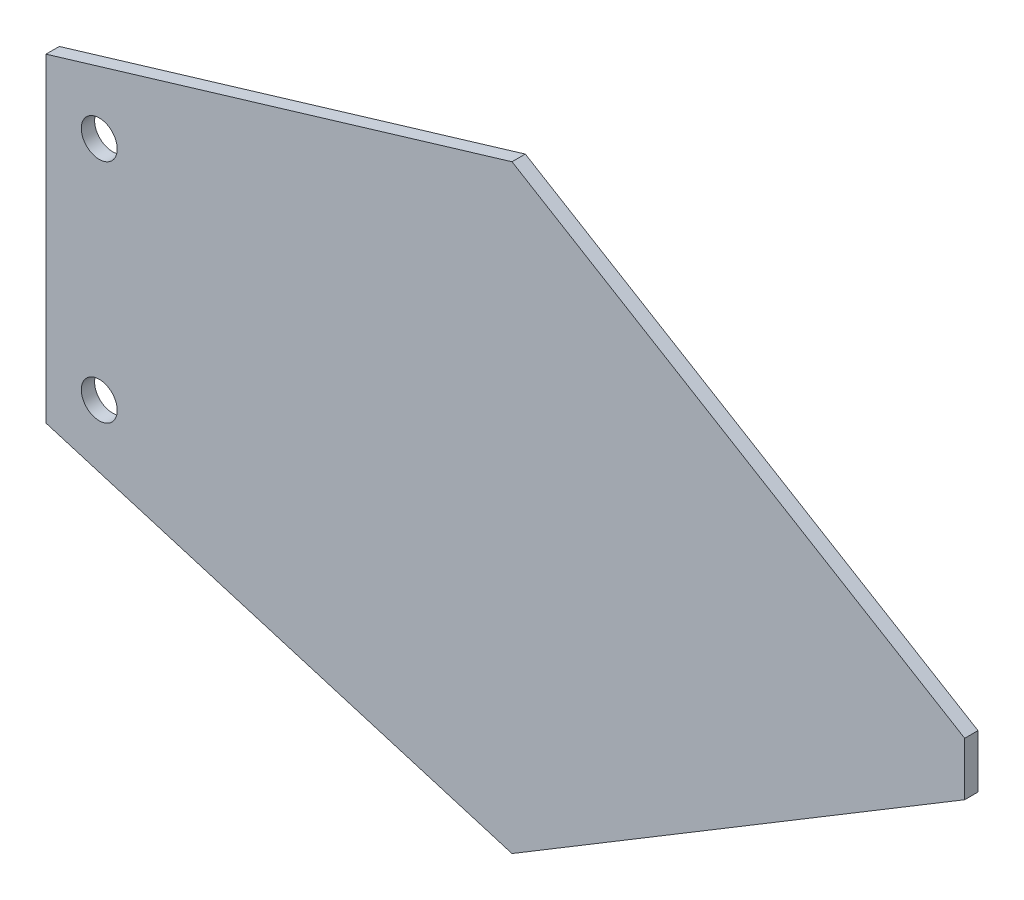
from build123d import *

# Parameters (mm, degrees)
SKETCH_1_W          = 690
SKETCH_1_H          = 450
EXTRUDE_1_DEPTH     = 10
SKETCH_2_R          = 13.5
CUT_EXTRUDE_1_DEPTH = 10


with BuildPart() as part:
    # 草图1 → 凸台-拉伸1 (new body)
    with BuildSketch(Plane.XY):
        Rectangle(SKETCH_1_W, SKETCH_1_H)
    extrude(amount=EXTRUDE_1_DEPTH)

    # 草图2 → 切除-拉伸1 (cut)
    with BuildSketch(Plane.XY.offset(10)):
        Polygon((-345, 225), (-345, 120), (5, 225), align=None)
        Polygon((345, 225), (5, 225), (345, 20), align=None)
        Polygon((345, -20), (5, -225), (345, -225), align=None)
        Polygon((5, -225), (-345, -120), (-345, -225), align=None)
        with Locations((-305, -85)):
            Circle(SKETCH_2_R)
        with Locations((-305, 85)):
            Circle(SKETCH_2_R)
    extrude(amount=-CUT_EXTRUDE_1_DEPTH, mode=Mode.SUBTRACT)


solid = part.part
